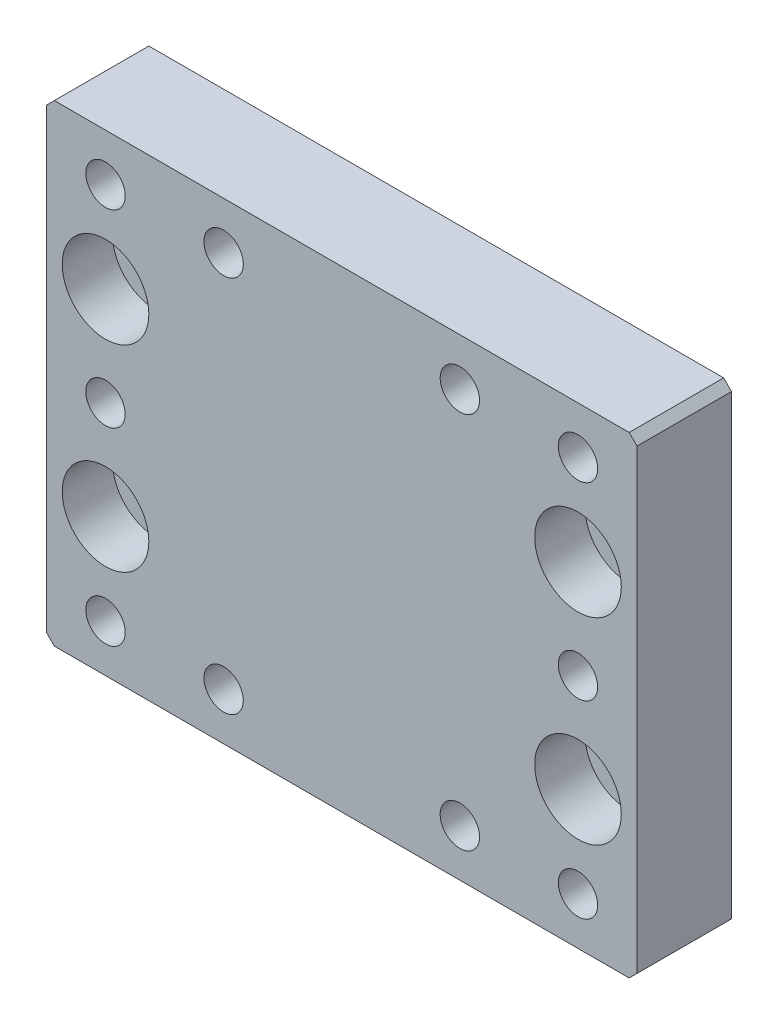
SolidWorks part; units mm, degrees
material "AL6061"
ref_plane "Front Plane" through (0, 0, 0) normal (0, 0, 1) x (1, 0, 0)
ref_plane "Top Plane" through (0, 0, 0) normal (0, 1, 0) x (1, 0, 0)
ref_plane "Right Plane" through (0, 0, 0) normal (1, 0, 0) x (0, 0, -1)
sketch "Sketch1" plane through (0, 0, 0) normal (0, 0, 1) x (1, 0, 0)
  line L1 (-37.5, 30) -> (37.5, 30)
  line L2 (-37.5, 30) -> (-37.5, -30)
  line L3 (-37.5, -30) -> (37.5, -30)
  line L4 (37.5, 30) -> (37.5, -30)
  line L5 (-37.5, 30) -> (37.5, -30) construction
  line L6 (-37.5, -30) -> (37.5, 30) construction
  point P0 (0, 0)
  dimension "D1" = 60
  dimension "D2" = 75
extrude "Boss-Extrude1" add sketch "Sketch1" along normal mid plane 12
hole_wizard "M6 Tapped Hole1" positions "Sketch4" profile "Sketch5" tap size "M6" standard "ISO" end condition through all
sketch "Sketch4" plane through (0, 0, 6) normal (0, 0, 1) x (1, 0, 0)
  point P0 (30, 24)
  point P3 (30, -24)
  point P6 (-30, -24)
  point P9 (-30, 24)
sketch "Sketch5" plane through (30, 24, 6) normal (1, 0, 0) x (0, -1, 0)
  line L0 (0, 0) -> (0, 12)
  line L1 (0, 12) -> (2.5, 12)
  line L2 (2.5, 12) -> (2.5, 0)
  line L5 (2.5, 0) -> (0, 0)
  line L11 (0, -6.35) -> (0, 107.95) construction
  dimension "通孔螺纹孔钻头直径" = 5
  dimension "通孔螺纹孔钻头深度" = 12
cosmetic thread "Cosmetic Thread1" parameters "D2"=6
cosmetic thread "Cosmetic Thread2" parameters "D2"=6
cosmetic thread "Cosmetic Thread3" parameters "D2"=6
cosmetic thread "Cosmetic Thread4" parameters "D2"=6
hole_wizard "CBORE for M6 Hex Socket Head Cap Screw1" positions "Sketch6" profile "Sketch7" counterbore size "M6" standard "ISO" end condition through all
sketch "Sketch6" plane through (0, 0, 6) normal (0, 0, 1) x (1, 0, 0)
  line L0 (0, 0) -> (0, 45.3835) construction
  line L1 (0, 0) -> (43.463, 0) construction
  point P0 (-30, 12.5)
  point P2 (30, 12.5)
  point P16 (-30, -12.5)
  point P18 (30, -12.5)
  dimension "D1" = 25
sketch "Sketch7" plane through (-30, 12.5, 6) normal (1, 0, 0) x (0, -1, 0)
  line L0 (0, 0) -> (0, 12)
  line L1 (0, 12) -> (3.3, 12)
  line L3 (3.3, 12) -> (3.3, 6.4)
  line L4 (3.3, 6.4) -> (5.5, 6.4)
  line L5 (5.5, 6.4) -> (5.5, 0)
  line L7 (5.5, 0) -> (0, 0)
  line L11 (0, -6.35) -> (0, 107.95) construction
  dimension "通孔孔直径" = 6.6
  dimension "通孔孔深度" = 12
  dimension "柱形沉头孔直径" = 11
  dimension "柱形沉头孔深度" = 6.4
hole_wizard "Blind Pin Hole3 (size mm)" positions "Sketch10" profile "Sketch11" hole size "Ø5.0" standard "ISO"
sketch "Sketch10" plane through (0, 0, 6) normal (0, 0, 1) x (1, 0, 0)
  point P0 (-30, 0)
  point P2 (30, 0)
sketch "Sketch11" plane through (-30, 0, 6) normal (1, 0, 0) x (0, -1, 0)
  line L0 (0, 0) -> (0, 12.5022)
  line L1 (0, 12.5022) -> (2.5, 11)
  line L2 (2.5, 11) -> (2.5, 0)
  line L5 (2.5, 0) -> (0, 0)
  line L10 (0, 12.5022) -> (-2.5, 11) construction
  line L11 (0, -6.35) -> (0, 107.95) construction
  dimension "孔直径" = 5
  dimension "孔深度" = 11
  dimension "导头角度" = 118
hole_wizard "大小mm 暗销孔3" positions "Sketch12" profile "Sketch13" hole size "Ø5.0" standard "ISO"
sketch "Sketch12" plane through (0, 0, 6) normal (0, 0, 1) x (1, 0, 0)
  line L0 (0, 0) -> (0, 43.9588) construction
  line L3 (0, 0) -> (50.3726, 0) construction
  point P0 (-15, 24)
  point P2 (15, -24)
  point P6 (15, 24)
  point P8 (-15, -24)
  dimension "D1" = 15
sketch "Sketch13" plane through (-15, 24, 6) normal (1, 0, 0) x (0, -1, 0)
  line L0 (0, 0) -> (0, 11.5022)
  line L1 (0, 11.5022) -> (2.5, 10)
  line L2 (2.5, 10) -> (2.5, 0)
  line L5 (2.5, 0) -> (0, 0)
  line L10 (0, 11.5022) -> (-2.5, 10) construction
  line L11 (0, -6.35) -> (0, 107.95) construction
  dimension "孔直径" = 5
  dimension "孔深度" = 10
  dimension "导头角度" = 118
chamfer "Chamfer1" distance 1 angle 45 4 edges at (-37.5, 30, 0) (-37.5, -30, 0) (37.5, -30, 0) (37.5, 30, 0)
